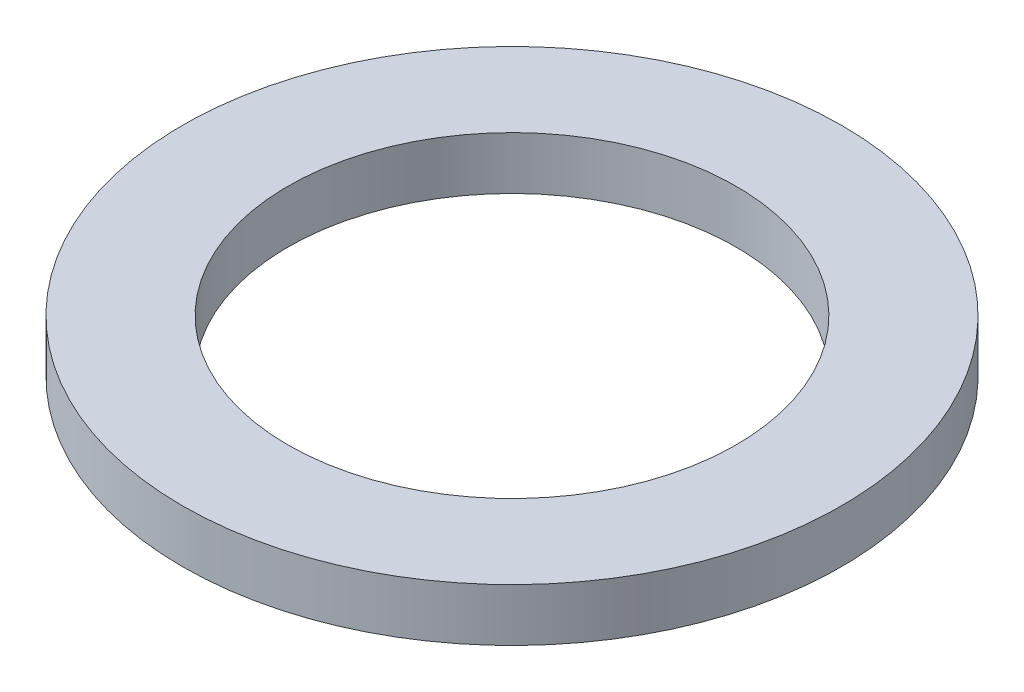
from build123d import *

# Parameters (mm, degrees)
SKETCH1_R           = 12.5
SKETCH1_R_2         = 8.5
BOSS_EXTRUDE1_DEPTH = 2


with BuildPart() as part:
    # Sketch1 → Boss-Extrude1 (new body)
    with BuildSketch(Plane(origin=(0, 0, 0), x_dir=(1, 0, 0), z_dir=(0, 1, 0))):
        with Locations(Location((0, 0, 0), (0, 0, 270))):
            Circle(SKETCH1_R)
        with Locations(Location((0, 0, 0), (0, 0, 270))):
            Circle(SKETCH1_R_2, mode=Mode.SUBTRACT)
    extrude(amount=BOSS_EXTRUDE1_DEPTH)


solid = part.part
